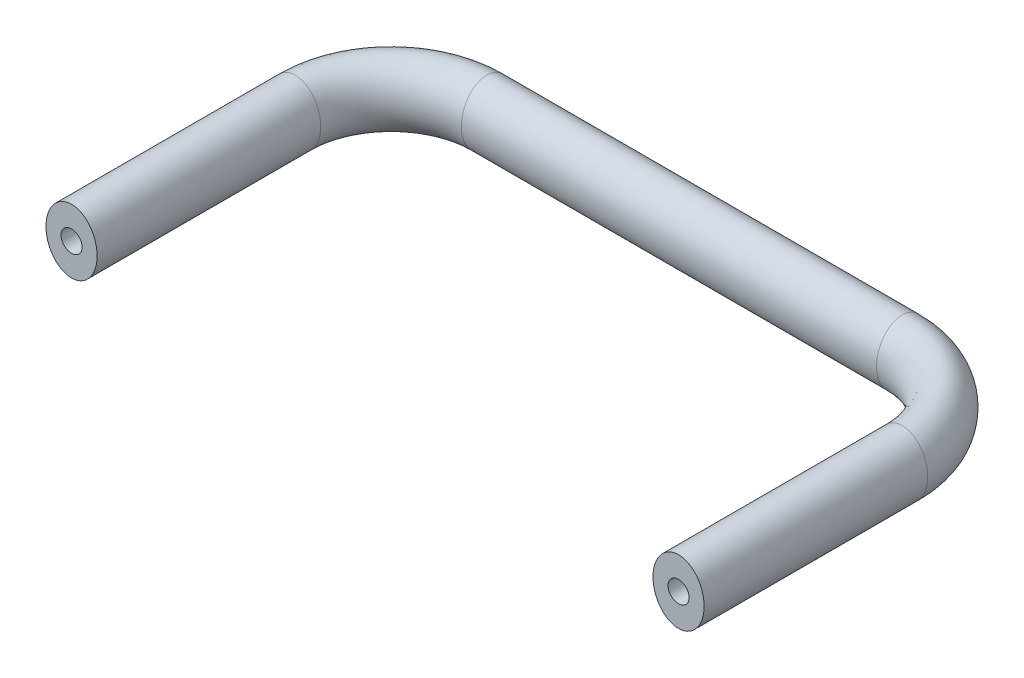
SolidWorks part; units mm, degrees
material "6061 合金"
ref_plane "前视基准面" through (0, 0, 0) normal (0, 0, 1) x (1, 0, 0)
ref_plane "上视基准面" through (0, 0, 0) normal (0, 1, 0) x (1, 0, 0)
ref_plane "右视基准面" through (0, 0, 0) normal (1, 0, 0) x (0, 0, -1)
sketch "草图1" plane through (0, 0, 0) normal (0, 0, 1) x (1, 0, 0)
  ellipse E0 centre (0, 0) end of major axis (0, 5) minor radius 4
  dimension "D1" = 8
  dimension "D2" = 10
sketch "草图2" plane through (0, 0, 0) normal (0, 1, 0) x (1, 0, 0)
  line L0 (0, 0) -> (0, 35)
  line L1 (15, 50) -> (80, 50)
  line L2 (95, 35) -> (95, 0)
  arc A0 (80, 50) -> (95, 35) centre (80, 35) cw
  arc A1 (0, 35) -> (15, 50) centre (15, 35) cw
  dimension "D3" = 15
  dimension "D1" = 95
  dimension "D2" = 50
sweep "扫描1" add profiles "草图1" path "草图2"
hole_wizard "M4 螺纹孔1" positions "草图7" profile "草图8" tap size "M4" standard "GB"
sketch "草图7" plane through (0, 0, 0) normal (0, 0, 1) x (1, 0, 0)
  point P0 (0, 0)
  point P3 (95, 0)
  dimension "D1" = 95
sketch "草图8" plane through (0, 0, 0) normal (1, 0, 0) x (0, -1, 0)
  line L0 (0, 0) -> (0, 12.4914)
  line L1 (0, 12.4914) -> (1.65, 11.5)
  line L2 (1.65, 11.5) -> (1.65, 0)
  line L5 (1.65, 0) -> (0, 0)
  line L10 (0, 12.4914) -> (-1.65, 11.5) construction
  line L11 (0, -6.35) -> (0, 107.95) construction
  dimension "螺纹孔钻头直径" = 3.3
  dimension "螺纹孔钻头深度" = 11.5
  dimension "导头角度" = 118
cosmetic thread "孔螺蚊线1" parameters "D1"=8, "D2"=4
cosmetic thread "孔螺蚊线2" parameters "D1"=8, "D2"=4
